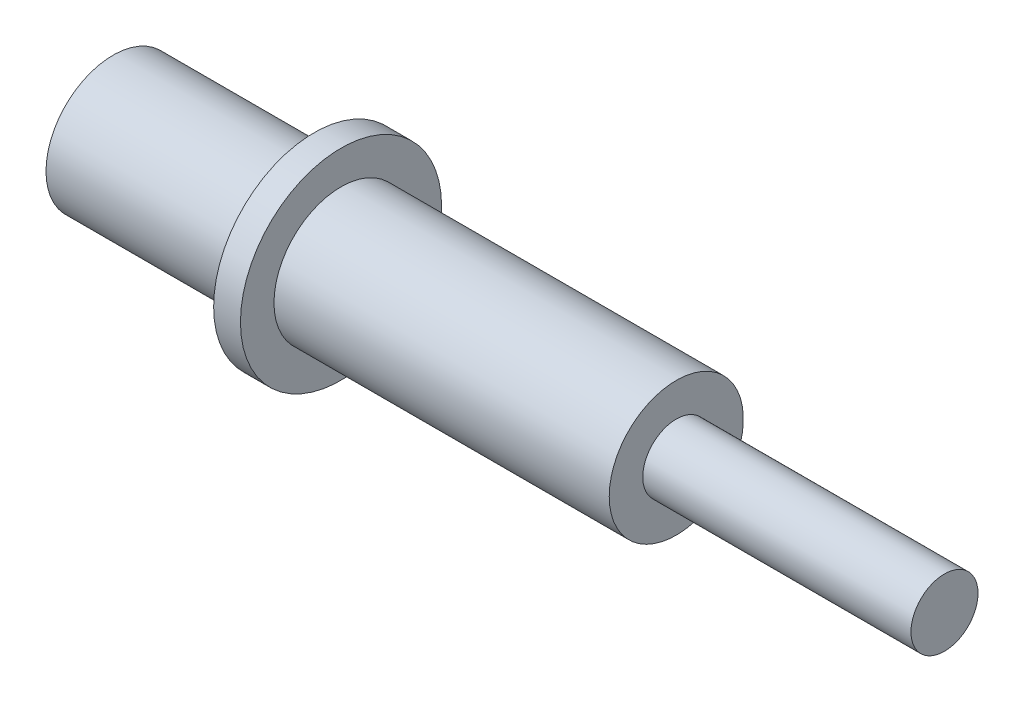
from build123d import *

# Parameters (mm, degrees)
SKETCH_1_R      = 2.5
EXTRUDE_1_DEPTH = 20
SKETCH_2_R      = 5
EXTRUDE_2_DEPTH = 25
SKETCH_3_R      = 7.5
EXTRUDE_3_DEPTH = 2
SKETCH_4_R      = 5
EXTRUDE_4_DEPTH = 15


with BuildPart() as part:
    # 草图1 → 凸台-拉伸1 (new body)
    with BuildSketch(Plane(origin=(0, 0, 0), x_dir=(0, 0, -1), z_dir=(1, 0, 0))):
        Circle(SKETCH_1_R)
    extrude(amount=EXTRUDE_1_DEPTH)

    # 草图2 → 凸台-拉伸2 (add)
    with BuildSketch(Plane.ZY):
        Circle(SKETCH_2_R)
    extrude(amount=EXTRUDE_2_DEPTH)

    # 草图3 → 凸台-拉伸3 (add)
    with BuildSketch(Plane.ZY.offset(25)):
        Circle(SKETCH_3_R)
    extrude(amount=EXTRUDE_3_DEPTH)

    # 草图4 → 凸台-拉伸4 (add)
    with BuildSketch(Plane.ZY.offset(27)):
        Circle(SKETCH_4_R)
    extrude(amount=EXTRUDE_4_DEPTH)


solid = part.part
